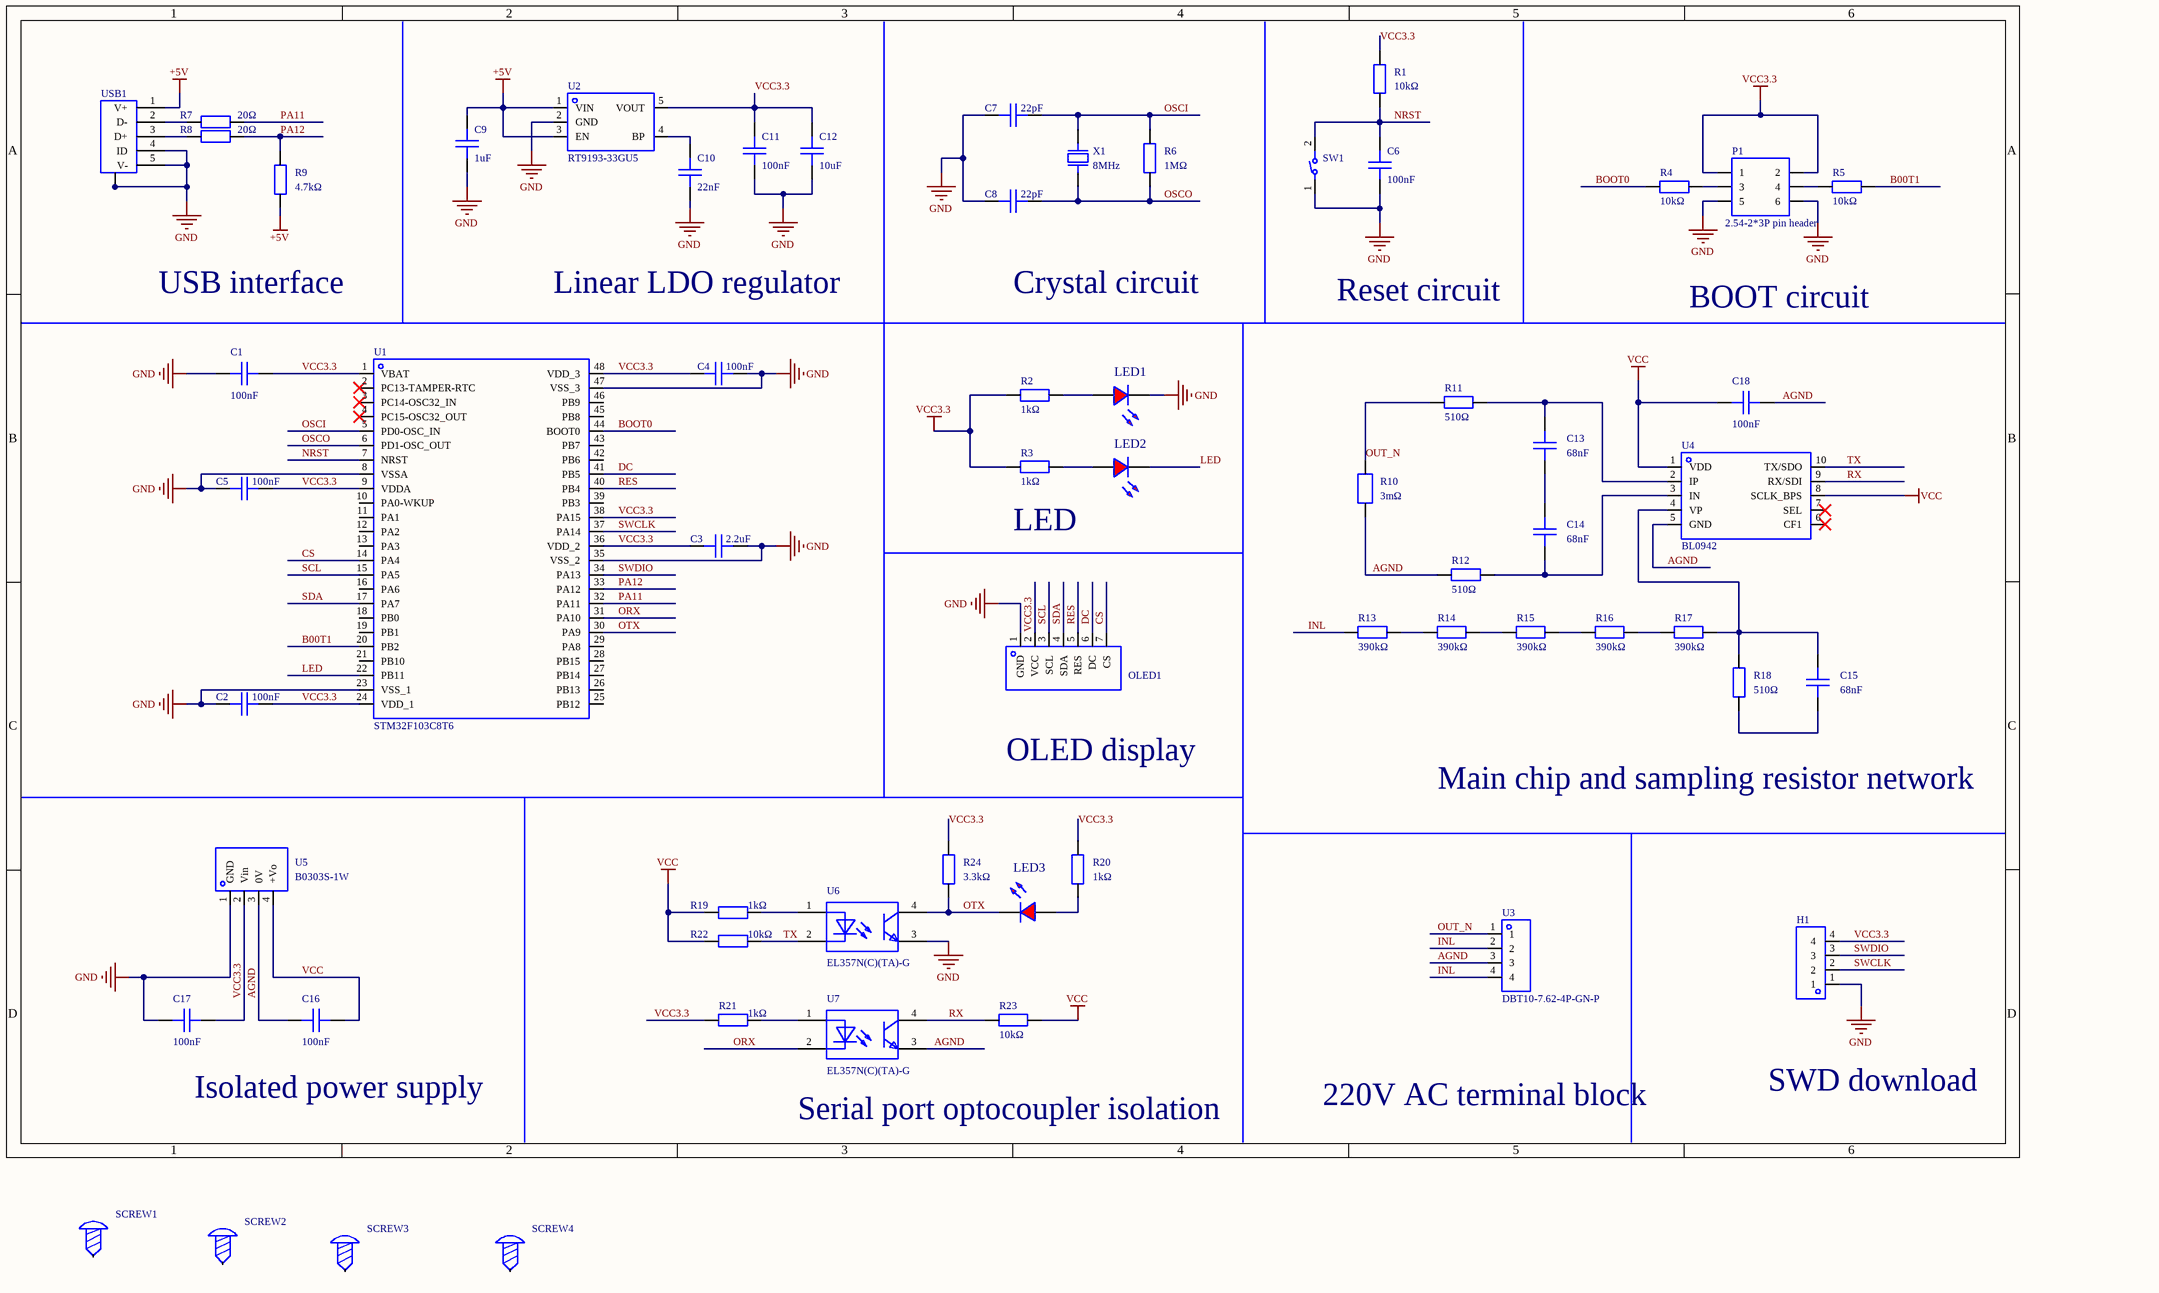
[diagram p0: MISC61948-3.schdoc]
# Altium project MISC61948-2.PrjPcb
1 sheet, 62 parts. Net scope: global (net labels, ports and power ports of the same name join across sheets).
Board file: MISC61948.pcbdoc

## Sheet MISC61948-3.schdoc
size 355 x 203 mm; Version: V1.0; @Project Name: MISC61948; @Update Date: 2026-05-21; @Create Date: 2026-05-21; @Board Name: MISC61948; @Create Time: 20:35:06; @Page Count: 1; @Page No: 1; @Schematic Name: MISC61948; @Update Time: 20:35:06; Size: A4

### Parts
C1  100nF  [CAP-SMD_L2.0-W1.25]
C2  100nF  [CAP-SMD_L2.0-W1.25]
C3  2.2uF  [C0805]
C4  100nF  [CAP-SMD_L2.0-W1.25]
C5  100nF  [CAP-SMD_L2.0-W1.25]
C6  100nF  [CAP-SMD_L2.0-W1.25]
C7  22pF  [C0805]
C8  22pF  [C0805]
C9  1uF  [C0805]
C10  22nF  [C0805]
C11  100nF  [CAP-SMD_L2.0-W1.25]
C12  10uF  [C0805]
C13  68nF  [C0805]
C14  68nF  [C0805]
C15  68nF  [C0805]
C16  100nF  [CAP-SMD_L2.0-W1.25]
C17  100nF  [CAP-SMD_L2.0-W1.25]
C18  100nF  [CAP-SMD_L2.0-W1.25]
H1  PZ254V-11-04P  [HDR-TH_4P-P2.54-V-M]  (value not drawn)
LED1  (no value)  [LED_0805]
LED2  (no value)  [LED_0805]
LED3  (no value)  [LED_0805]
OLED1  HS96L01W4S03  [OLED-TH_HS96L01W4S03]  (value not drawn)
P1  2.54-2*3P pin header  [IDC-TH_6P-P2.54_C11214]
R1  10kΩ  [R0805]
R2  1kΩ  [R0805]
R3  1kΩ  [R0805]
R4  10kΩ  [R0805]
R5  10kΩ  [R0805]
R6  1MΩ  [R0805]
R7  20Ω  [R0805]
R8  20Ω  [R0805]
R9  4.7kΩ  [R0805]
R10  3mΩ  [R2512]
R11  510Ω  [R0805]
R12  510Ω  [R0805]
R13  390kΩ  [R0805]
R14  390kΩ  [R0805]
R15  390kΩ  [R0805]
R16  390kΩ  [R0805]
R17  390kΩ  [R0805]
R18  510Ω  [R0805]
R19  1kΩ  [R0805]
R20  1kΩ  [R0805]
R21  1kΩ  [R0805]
R22  10kΩ  [R0805]
R23  10kΩ  [R0805]
R24  3.3kΩ  [R0805]
SCREW1  (no value)  [M3螺丝]
SCREW2  (no value)  [M3螺丝]
SCREW3  (no value)  [M3螺丝]
SCREW4  (no value)  [M3螺丝]
SW1  TS1305-TZ43HBM  [SW-SMD_L6.0-W3.5-LS8.0_TS04-TBW1FH4.3]  (value not drawn)
U1  STM32F103C8T6  [LQFP-48_L7.0-W7.0-P0.50-LS9.0-BL]
U2  RT9193-33GU5  [SC-70-5_L2.0-W1.3-P0.65-LS2.1-BL]
U3  DBT10-7.62-4P-GN-P  [CONN-TH_DBT10-7.62-4P]
U4  BL0942  [SSOP-10_L4.9-W3.9-P1.00-LS6.0-BL]
U5  B0303S-1W  [PWRM-TH_BXXXXS-1W]
U6  EL357N(C)(TA)-G  [OPTO-SMD-4_L4.4-W4.1-P2.54-LS7.0-TL]
U7  EL357N(C)(TA)-G  [OPTO-SMD-4_L4.4-W4.1-P2.54-LS7.0-TL]
USB1  920-E52A2021S10100  [MICRO-USB-SMD_5P-P0.65-H-F_C10418]  (value not drawn)
X1  8MHz  [CRYSTAL-SMD_L11.4-W4.7-LS12.7]

### Nets
+5V: C9.2 R9.1 U2.1(VIN) U2.3(EN) USB1.1(V+)
GND: C1.1 C2.1 C3.2 C4.1 C5.1 C6.2 C7.2 C8.2 C9.1 C10.1 C11.2 C12.1 C17.1 H1.1 LED1.1(C) OLED1.1(GND) P1.5 P1.6 SW1.1 U1.8(VSSA) U1.23(VSS_1) U1.35(VSS_2) U1.47(VSS_3) U2.2(GND) U5.1(GND) U6.3 USB1.4(ID) USB1.5(V-) USB1.SH0(MTN) USB1.SH1 USB1.SH2 USB1.SH3
VCC: C16.2 C18.1 R19.2 R22.2 R23.2 U4.1(VDD) U4.8(SCLK_BPS) U5.4(+Vo)
VCC3.3: C1.2 C2.2 C3.1 C4.2 C5.2 C11.1 C12.2 C17.2 H1.4 OLED1.2(VCC) P1.1 P1.2 R1.2 R2.2 R3.2 R20.1 R21.2 R24.1 U1.1(VBAT) U1.9(VDDA) U1.24(VDD_1) U1.36(VDD_2) U1.38(PA15) U1.48(VDD_3) U2.5(VOUT) U5.2(Vin)
AGND: C16.1 C18.2 R10.1 R12.2 U3.3 U4.5(GND) U5.3(0V) U7.3
B00T1: R5.1 U1.20(PB2)
BOOT0: R4.2 U1.44(BOOT0)
CS: OLED1.7(CS) U1.14(PA4)
DC: OLED1.6(DC) U1.41(PB5)
INL: R13.2 U3.2 U3.4
LED: LED2.1(C) U1.22(PB11)
NRST: C6.1 R1.1 SW1.2 U1.7(NRST)
ORX: U1.31(PA10) U7.2
OSCI: C7.1 R6.2 U1.5(PD0-OSC_IN) X1.2(OSC2)
OSCO: C8.1 R6.1 U1.6(PD1-OSC_OUT) X1.1(OSC1)
OTX: LED3.1(C) R24.2 U1.30(PA9) U6.4
OUT_N: R10.2 R11.2 U3.1
PA11: R7.2 U1.32(PA11)
PA12: R8.2 R9.2 U1.33(PA12)
RES: OLED1.5(RES) U1.40(PB4)
RX: R23.1 U4.9(RX/SDI) U7.4
SCL: OLED1.3(SCL) U1.15(PA5)
SDA: OLED1.4(SDA) U1.17(PA7)
SWCLK: H1.2 U1.37(PA14)
SWDIO: H1.3 U1.34(PA13)
TX: R22.1 U4.10(TX/SDO) U6.2
NetC10_2: C10.2 U2.4(BP)
NetC13_1: C13.1 R11.1 U4.2(IP)
NetC13_2: C13.2 C14.1
NetC14_2: C14.2 R12.1 U4.3(IN)
NetC15_1: C15.1 R17.1 R18.1 U4.4(VP)
NetC15_2: C15.2 R18.2
NetLED1_2: LED1.2(A) R2.1
NetLED2_2: LED2.2(A) R3.1
NetLED3_2: LED3.2(A) R20.2
NetP1_3: P1.3 R4.1
NetP1_4: P1.4 R5.2
NetR7_1: R7.1 USB1.2(D-)
NetR8_1: R8.1 USB1.3(D+)
NetR13_1: R13.1 R14.2
NetR14_1: R14.1 R15.2
NetR15_1: R15.1 R16.2
NetR16_1: R16.1 R17.2
NetR19_1: R19.1 U6.1
NetR21_1: R21.1 U7.1

Not connected (* = marked no-connect by the designer): SCREW1 1; SCREW2 1; SCREW3 1; SCREW4 1; U1 2(PC13-TAMPER-RTC)* 3(PC14-OSC32_IN)* 4(PC15-OSC32_OUT)* 10(PA0-WKUP) 11(PA1) 12(PA2) 13(PA3) 16(PA6) 18(PB0) 19(PB1) 21(PB10) 25(PB12) 26(PB13) 27(PB14) 28(PB15) 29(PA8) 39(PB3) 42(PB6) 43(PB7) 45(PB8) 46(PB9); U4 6(CF1)* 7(SEL)*

### Notes on the sheet
- USB interface
- Linear LDO regulator
- Crystal circuit
- Reset circuit
- BOOT circuit
- (near R3) LED
- OLED display
- Main chip and sampling resistor network
- Isolated power supply
- 220V AC terminal block
- SWD download
- (near U7) Serial port optocoupler isolation

### Library data of the parts
C1 C2 C4-C6 C11 C16-C18 = FCC0805B104K500DT: Capacitance: 100nF;Tolerance: ±10%;Rated voltage: 50V;Temperature coefficient: X7R;; Manufacturer: FOJAN(富捷); AddInBom: yes; ModelId: dce19e309e9b4209af79576cb8c62f2f0819f05c4eef4c71ace90d822a990e87; ModelName: CAP-SMD_L2.0-W1.3-H1.3; ModelTransform: 78.74,49.2125,0,0,0,0,0,0,0; Symbol: FCC0805B104K500DT; Device: FCC0805B104K500DT; LCSC Part Name: 100nF ±10% 50V; SupplierPart: C5137467; ManufacturerPart: FCC0805B104K500DT; Supplier Footprint: 0805; JLCPCB Part Class: Extended Part; Datasheet: https://item.szlcsc.com/datasheet/FCC0805B104K500DT/5746969.html; Supplier: LCSC; ConvertToPcb: yes; FootprintName: CAP-SMD_L2.0-W1.25; Value: 100nF; Tolerance: ±10%; Voltage Rating: 50V; Temperature Coefficient: X7R
C3 C7-C10 C12-C15 = CAP_0805: Symbol: Capacitance; ConvertToPcb: yes; ModelId: 1ba041120af144c991958decab20d2410819f05c4eef4c71ace90d822a990e87; ModelName: C0805_L2.0-W1.3-H1.3; ModelTransform: 78.74,51.181,0,0,0,0,0,0.0005,0; Device: CAP_0805; AddInBom: yes; Supplier Footprint: 0805; FootprintName: C0805
  C3: Value: 2.2uF
  C7 C8: Value: 22pF
  C9: Value: 1uF
  C10: Value: 22nF
  C12: Value: 10uF
  C13-C15: Value: 68nF
H1 = PZ254V-11-04P: 插针结构:1x4P;间距:2.54mm;行距:-;圆针/方针:方针;安装方式:直插;排数:单排;总PIN位数:4P;额定电流:3A;额定电压:250V;配合针长度:6mm;塑高:2.5mm;端接针长度:3mm;触头材质:-;工作温度:-40℃~+105℃;颜色:黑色;; Manufacturer: XFCN(兴飞); Symbol: PZ254V-11-04P_C2691448; AddInBom: yes; ModelId: 112f4d05e8d64e99ab9a333894bea4f90819f05c4eef4c71ace90d822a990e87; ModelName: HDR-TH_4P-P2.54-M-LI-1X4P; ModelTransform: 399.999,104.7242,0,0,0,0,0,0,-118.11; Pin Structure: 1x4P; Pitch: 2.54mm; Circluar Pins/Square Pins: Square pin; Current Rating: 3A; Voltage Rating (Max): 250V; Device: PZ254V-11-04P; LCSC Part Name: 1x4P 间距:2.54mm 方针 直插; SupplierPart: C2691448; ManufacturerPart: PZ254V-11-04P; Supplier Footprint: 插件,P=2.54mm; JLCPCB Part Class: Extended Part; Datasheet: https://item.szlcsc.com/datasheet/PZ254V-11-04P/2801085.html; Supplier: LCSC; ConvertToPcb: yes; FootprintName: HDR-TH_4P-P2.54-V-M; Row Spacing: -; Mounting Type: Through-hole; Number of Rows: Single row; Number of Pins: 4P; Length of Mating Pin: 6mm; Insulation Height: 2.5mm; Length of End Connection Pin: 3mm; Contact Material: -; Operating Temperature: -40℃~+105℃; Color: Black
LED1-LED3 = LED_0805-R: Symbol: LED_R; Convert to PCB: yes; 3D Model: 33fb9fca58e84f37a403ebeef4c28b770819f05c4eef4c71ace90d822a990e87; 3D Model Transform: 78.7,49.1,39.3,0,0,0,0,0,0; ModelName: LED-0805_R; Device: LED_0805-R; Add into BOM: yes; Supplier Footprint: 0805; FootprintName: LED_0805
OLED1 = HS96L01W4S03: Size (inch): 0.96;Pixel resolution: 128x64;; Manufacturer: HS(汉昇); AddInBom: yes; ModelId: 7927fe0e3c8842749d8ccfcaf6d2f4920819f05c4eef4c71ace90d822a990e87; ModelTransform: 1074.801,1094.486,0,0,0,0,0,-488.188,-157.48; Type of Drive: Passive (PMOLED); Display Range: 21.74x10.86mm; Display Color: White; Luminance: 100cd/m2; Quiescent Current: 5uA; Symbol: HS96L01W4S03; Device: HS96L01W4S03; LCSC Part Name: 0.96寸 白光 128x64像素分辨率; SupplierPart: C5139758; ManufacturerPart: HS96L01W4S03; Supplier Footprint: -; JLCPCB Part Class: Extended Part; Datasheet: https://item.szlcsc.com/datasheet/HS96L01W4S03/5751920.html; Supplier: LCSC; ConvertToPcb: yes; FootprintName: OLED-TH_HS96L01W4S03; ModelName: OLED-TH_HS96L01W4S03; Size: 0.96; Dot Pixels: 128x64; Operating Temperature: -40℃~+80℃
P1 = 2.54-2*3P简牛: 连接器类型:简牛座;间距:2.54mm;结构:2x3P;额定电流:1A;安装方式:直插;行距:2.54mm;排数:2;每排PIN数:3;触头材质:黄铜;触头镀层:金;工作温度:-55℃~+105℃;; Manufacturer: BOOMELE(博穆精密); Symbol: HDR-IDC-2.54-2X3P; AddInBom: yes; ModelId: 8d5872ccea434d338d7c3a1455fd18c80819f05c4eef4c71ace90d822a990e87; ModelTransform: 599.999,348.41478,0,0,0,0,0.591,0.512,-137.795; Pitch: 2.54mm; Number of Positions or Pins: 2x3P; Current Rating: 1A; Holder Type: Through-hole; Number of PINs Per Row: 3; Device: 2.54-2*3P pin header; LCSC Part Name: 2.54mm 2x3P 排数:2 每排P数:3; SupplierPart: C11214; ManufacturerPart: 2.54-2*3P简牛; Supplier Footprint: 插件,P=2.54mm; JLCPCB Part Class: Extended Part; Datasheet: https://item.szlcsc.com/datasheet/2.54-2*3P%25E7%25AE%2580%25E7%2589%259B/11763.html; Supplier: LCSC; ConvertToPcb: yes; FootprintName: IDC-TH_6P-P2.54_C11214; ModelName: HDR-IDC-2.54-2X3P; Connector Type: Pin header; Row Spacing: 2.54mm; Number of Rows: 2; Contact Material: Brass; Contact Plating: Gold; Operating Temperature: -55℃~+105℃; Color: Black
R1-R9 R11-R24 = Res_0805: Symbol: Resistor; ConvertToPcb: yes; ModelId: 37a81e68749a4138bd2dfa6897b24b850819f05c4eef4c71ace90d822a990e87; ModelName: R0805_L2.0-W1.3-H0.6; ModelTransform: 78.74,51.181,0,0,0,0,0,-0.0005,0; Device: Res_0805; AddInBom: yes; Supplier Footprint: 0805; FootprintName: R0805
  R1 R4 R5 R22 R23: Value: 10kΩ
  R2 R3 R19-R21: Value: 1kΩ
  R6: Value: 1MΩ
  R7 R8: Value: 20Ω
  R9: Value: 4.7kΩ
  R11 R12 R18: Value: 510Ω
  R13-R17: Value: 390kΩ
  R24: Value: 3.3kΩ
R10 = JER2512F3R003L: Resistor type: sampling resistor; alloy resistor;Resistance: 3mΩ;Tolerance: ±1%;Power: 3W;Temperature coefficient: ±50ppm/℃;; Manufacturer: JIERR(捷而瑞); AddInBom: yes; ModelId: 954b67263d9e4f3582d8de3f8c8464210819f05c4eef4c71ace90d822a990e87; ModelName: R2512_L6.3-W3.2-H0.6; ModelTransform: 248.031,125.984,0,0,0,0,-0.0005,0,0; Symbol: JER2512F3R003L; Device: JER2512F3R003L; LCSC Part Name: 3mΩ 3W 2512 ±1%; SupplierPart: C46634457; ManufacturerPart: JER2512F3R003L; Supplier Footprint: 2512; JLCPCB Part Class: Extended Part; Datasheet: https://item.szlcsc.com/datasheet/JER2512F3R003L/48788259.html; Supplier: LCSC; ConvertToPcb: yes; FootprintName: R2512; Type: Sampling resistor; alloy resistor; Value: 3mΩ; Tolerance: ±1%; Power(Watts): 3W; Temperature Coefficient: ±50ppm/℃
SCREW1-SCREW4 = M3螺丝: Symbol: Screw hole; Device: M3 screw; ConvertToPcb: yes; AddInBom: yes; Supplier Footprint: 插件; FootprintName: M3 screw
SW1 = TS1305-TZ43HBM: 电路结构:单刀单掷;按钮形状:矩形按钮;安装方式:立贴;开关长度:6mm;开关宽度:3.5mm;开关高度:4.3mm;带支架:不带支架;触点电流:50mA;额定电压:12V;带灯:无;; Manufacturer: BXCONN(宝讯); AddInBom: yes; ModelId: 01d898389ac64b298c2b5578d6434a870819f05c4eef4c71ace90d822a990e87; ModelTransform: 314.96,138.1887,0,0,0,0,-0.51,0,0; Circuit: SPST; Actuator Style: Rectangular button; Switch Height: 4.3mm; with Bracket: Without bracket; Contact Current: 50mA; Voltage Rating: 12V; Actuator/Cap Color: White; With Lamp: None; Symbol: TS1305-TZ43HBM; Device: TS1305-TZ43HBM; LCSC Part Name: 3*6*4.3  立贴   轻触开关; SupplierPart: C36936593; ManufacturerPart: TS1305-TZ43HBM; Supplier Footprint: SMD,6x3.5mm; JLCPCB Part Class: Extended Part; Datasheet: https://item.szlcsc.com/datasheet/TS1305-TZ43HBM/38663669.html; Supplier: LCSC; ConvertToPcb: yes; FootprintName: SW-SMD_L6.0-W3.5-LS8.0_TS04-TBW1FH4.3; ModelName: SW-SMD_L6.0-W3.5-LS8.0_TS04-TBW1FH4.3; Mounting Type: Vertical SMD; Length: 6mm; Width: 3.5mm; Termination Style: Gull-wing
U1 = STM32F103C8T6: CPU core: ARM-M3;CPU max frequency: 72MHz;Application field: -;; Manufacturer: ST(意法半导体); AddInBom: yes; ModelId: 093be70396ff421eb2cdb946d5311efc0819f05c4eef4c71ace90d822a990e87; ModelName: LQFP-48_L7.0-W7.0-H1.4-LS9.0-P0.50; ModelTransform: 354.331,354.331,0,0,0,0,0,0,0; Program Storage Size: 64KB; Program Memory Type: FLASH; Number of I/O: 37; ADC (Bit): 12bit; Voltage - Supply: 2V~3.6V; Symbol: STM32F103C8T6; Device: STM32F103C8T6; LCSC Part Name: 主流增强型ARM Cortex-M3 MCU，具有64 KB Flash、72 MHz CPU、电机控制、USB和CAN; SupplierPart: C8734; ManufacturerPart: STM32F103C8T6; Supplier Footprint: LQFP-48(7x7); JLCPCB Part Class: Extended Part; Datasheet: https://item.szlcsc.com/datasheet/STM32F103C8T6/9243.html; Supplier: LCSC; ConvertToPcb: yes; FootprintName: LQFP-48_L7.0-W7.0-P0.50-LS9.0-BL; CPU Core: ARM-M3; CPU Maximum Speed: 72MHz; Applications: -
U2 = RT9193-33GU5: Output type: fixed;Operating voltage: 5.5V;Output voltage: 3.3V;Output current: 300mA;PSRR: 70dB@(100Hz);Output polarity: positive;; Manufacturer: RICHTEK(立锜); AddInBom: yes; ModelId: 180ad2a85d044b18a9defb4b28abe5600819f05c4eef4c71ace90d822a990e87; ModelTransform: 78.74,86.614,0,0,0,0,-0.002,0.001,0; Voltage Dropout: 220mV@(300mA); standby current: 90uA; Noise: 100uVrms; Number of Outputs: 1; Symbol: RT9193-33GU5; Device: RT9193-33GU5; LCSC Part Name: 3.3V 300mA 5.5V; SupplierPart: C425797; ManufacturerPart: RT9193-33GU5; Supplier Footprint: SC-70-5; JLCPCB Part Class: Extended Part; Datasheet: https://item.szlcsc.com/datasheet/RT9193-33GU5/419424.html; Supplier: LCSC; ConvertToPcb: yes; FootprintName: SC-70-5_L2.0-W1.3-P0.65-LS2.1-BL; ModelName: SC-70-5_L2.0-W1.3-P0.65-LS2.1-BL; Output Type: Fixed; Voltage - Supply: 5.5V; Output Voltage: 3.3V; Output Current: 300mA; Power Supply Rejection Ratio (PSRR): 70dB@(100Hz); Features: Overcurrent protection; overtemperature protection; Operating Temperature: -40℃~+85℃@(Ta); Output Configuration: Positive
U3 = DBT10-7.62-4P-GN-P: 隔板类型:两面;间距:7.62mm;结构:1x4P;安装方式:直插;引脚位置:边脚;排数:1;每排PIN数:4;额定电流:24A;额定电压:450V;线规 - AWG:14~22;线规 - 平方毫米:-;工作温度:-40℃~+105℃;颜色:绿色;; Manufacturer: DORABO(地博电气); AddInBom: yes; ModelId: 1d2b77d4cf214f9ab09439e281b7d9ba0819f05c4eef4c71ace90d822a990e87; ModelName: CONN-TH_WJ7.62-LI-4P-DBT10; ModelTransform: 1227.55664,488.188,0,0,0,0,-19.685,-145.669,-137.795; Barrier Type: Double-sided; Pitch: 7.62mm; Number of Positions or Pins: 1x4P; Pin Location: Side pins; Number of PINs Per Row: 4; Current Rating: 24A; Voltage Rating (Max): 450V; Wire Gauge - AWG: 14~22; Symbol: DBT10-7.62-4P; Device: DBT10-7.62-4P-GN-P; LCSC Part Name: 7.62mm 1x4P 直插 边脚 排数:1 每排P数:4; SupplierPart: C424698; ManufacturerPart: DBT10-7.62-4P-GN-P; Supplier Footprint: 插件,P=7.62mm; JLCPCB Part Class: Extended Part; Datasheet: https://item.szlcsc.com/datasheet/DBT10-7.62-4P-GN-P/418367.html; Supplier: LCSC; ConvertToPcb: yes; FootprintName: CONN-TH_DBT10-7.62-4P; Mounting Type: Through-hole; Number of Pins: 4P; Number of Rows: 1; Wire Gauge - mm2: -; Operating Temperature: -40℃~+105℃; Color: Green
U4 = BL0942_C2837510: BL0942 is an energy metering chip with built-in clock and no calibration required, suitable for single-phase multifunction energy meters, smart sockets, smart home appliances and similar applications, with high cost-effectiveness.; Manufacturer: BL(上海贝岭); AddInBom: yes; ModelId: d633480e87ce4338a1764e9c79a3c6ca0819f05c4eef4c71ace90d822a990e87; ModelName: SSOP-10_L4.9-W3.9-H1.5-LS6.0-P1.00; ModelTransform: 228.57954,188.976,0,90,0,0,0,0,0; Symbol: BL0942; Device: BL0942_C2837510; LCSC Part Name: BL0942内置时钟免校准计量芯片; SupplierPart: C2837510; ManufacturerPart: BL0942; Supplier Footprint: SSOP-10-150mil; JLCPCB Part Class: Extended Part; Datasheet: https://atta.szlcsc.com/upload/public/pdf/source/20220627/BFAD44701CA6DE9A8853C5A4834B6884.pdf; Supplier: LCSC; ConvertToPcb: yes; FootprintName: SSOP-10_L4.9-W3.9-P1.00-LS6.0-BL
U5 = B0303S-1W_C5280457: Size (mm): length 11.6 * width 6.0 * height 10.0; Manufacturer: NYBOXING(尼博星); AddInBom: yes; ModelId: baa693b409474499a66bc36dbe95a9430819f05c4eef4c71ace90d822a990e87; ModelTransform: 456.692,236.22,0,0,0,0,0,82.677,-137.795; Number of Outputs: 1; Voltage - Supply: 2.97V~3.63V; Output Voltage: 3.3V; Output Current(Max): 300mA; Conversion Efficiency: 81%; Capacitive Load(Max): 10uF; Switching Frequency: 100kHz; Ripple Noise: 75mVp-p; Symbol: B0303S-1W_C5280457; Device: B0303S-1W_C5280457; LCSC Part Name: 2.97V~3.63V 3.3V 1W; SupplierPart: C5280457; ManufacturerPart: B0303S-1W; Supplier Footprint: SIP,11.6x6mm; JLCPCB Part Class: Extended Part; Datasheet: https://item.szlcsc.com/datasheet/B0303S-1W/6016195.html; Supplier: LCSC; ConvertToPcb: yes; FootprintName: PWRM-TH_BXXXXS-1W; ModelName: PWRM-TH_BXXXXS-1W; Length: 11.6mm; Width: 6mm; Height: 10mm; Operating Temperature Range: -40℃~+85℃
U6 U7 = EL357N(C)(TA)-G_C42379244: 输入类型:DC;正向压降(Vf):1.2V;输出电流:50mA;隔离电压(Vrms):3.75kV;直流反向耐压(Vr):6V;负载电压:80V;输出通道数:1;集射极饱和电压(VCE(sat)):200mV@20mA,1mA;; Manufacturer: EVERLIGHT(亿光); AddInBom: yes; ModelId: f42cca50e4b4465cbb82017a511efd450819f05c4eef4c71ace90d822a990e87; ModelName: OPTO-SMD-4P_L4.1-W4.4-H2.0-LS7.0-P2.54; ModelTransform: 275.59,161.417,0,0,0,0,0,0,0; Input type: DC; Output Type: Phototransistor; Voltage - Forward(Vf): 1.2V; Output Current: 50mA; Isolation Voltage(Vrms): 3.75kV; Reverse Voltage: 6V; Load Voltage: 80V; Number of Outputs: 1; Rise time: 3us; Fall time: 4us; Current Transfer Ratio (CTR) Minimum: 200%; Current Transfer Ratio (CTR) Maximum/Saturation Value: 400%; Total Power Dissipation(Pd): 200mW; Symbol: EL357N(C)(TA)-G_C42379244; Device: EL357N(C)(TA)-G_C42379244; LCSC Part Name: DC 3.75kV; SupplierPart: C42379244; ManufacturerPart: EL357N(C)(TA)-G; Supplier Footprint: SOP-4-2.54mm; JLCPCB Part Class: Extended Part; Datasheet: https://www.everlighteurope.com/custom/files/datasheets/DPC-0000014.pdf; Supplier: LCSC; ConvertToPcb: yes; FootprintName: OPTO-SMD-4_L4.4-W4.1-P2.54-LS7.0-TL; Vce Saturation(VCE(sat)): 200mV@20mA,1mA; Operating Temperature: -55℃~+110℃; Forward Current(If): 50mA
USB1 = 920-E52A2021S10100: Connector type: Micro-B;Protocol standard: USB 2.0;Gender: female;Mounting: horizontal SMD;Contacts: 5P;Ports: 1;Rated current - power: 1A;Operating temperature: -30℃~+80℃;; Manufacturer: 精拓金; Symbol: micro USBFemale; AddInBom: yes; ModelId: 8d98bdb22dfe41cea8df3303517703a80819f05c4eef4c71ace90d822a990e87; ModelTransform: 315.054,220.472,0,180,0,0,0,-51.038,-39.37; Protocol Standard: USB 2.0; Number of Ports: 1; Detection color: Black; Device: 920-E52A2021S10100; LCSC Part Name: Micro-B 母 卧贴; SupplierPart: C10418; ManufacturerPart: 920-E52A2021S10100; Supplier Footprint: SMD; JLCPCB Part Class: Extended Part; Datasheet: https://item.szlcsc.com/datasheet/920-E52A2021S10100/10961.html; Supplier: LCSC; ConvertToPcb: yes; FootprintName: MICRO-USB-SMD_5P-P0.65-H-F_C10418; ModelName: MICRO-USB-SMD_5P-P0.65-H-F_C10418; Connector Type: Micro-B; Gender: Female; Mounting Type: Horizontal SMD; Number of Contacts: 5P; Current Rating-Power: 1A; Length: 5.15mm; Operating Temperature: -30℃~+80℃
X1 = X49SS2-8.000-F20JGDT: Crystal type: SMD crystal;Frequency: 8MHz;Frequency deviation at room temperature: ±30ppm;Load capacitance: 20pF;Frequency stability: ±50ppm;; Manufacturer: HCI(杭晶); AddInBom: yes; ModelId: be19d32e6d024fb4863eb8f4e3f5efcc0819f05c4eef4c71ace90d822a990e87; ModelTransform: 499.999,185.039,0,0,0,0,0,0,0; Equivalent Series Resistance(ESR): 60Ω; Symbol: X49SS2-8.000-F20JGDT; Device: X49SS2-8.000-F20JGDT; LCSC Part Name: HC-49SMD 2P 8MHz 20pF ±30ppm -40~+85℃(±50ppm); SupplierPart: C2842263; ManufacturerPart: X49SS2-8.000-F20JGDT; Supplier Footprint: HC-49SMD-2P; JLCPCB Part Class: Extended Part; Datasheet: https://item.szlcsc.com/datasheet/X49SS2-8.000-F20JGDT/3026537.html; Supplier: LCSC; ConvertToPcb: yes; FootprintName: CRYSTAL-SMD_L11.4-W4.7-LS12.7; ModelName: CRYSTAL-SMD_L11.4-W4.7-LS12.7; Type: SMD crystal; Value: 8MHz; Normal temperature Frequency Tolerance: ±30ppm; Load Capacitance: 20pF; Frequency Stability: ±50ppm; Operating Temperature: -40℃~+85℃